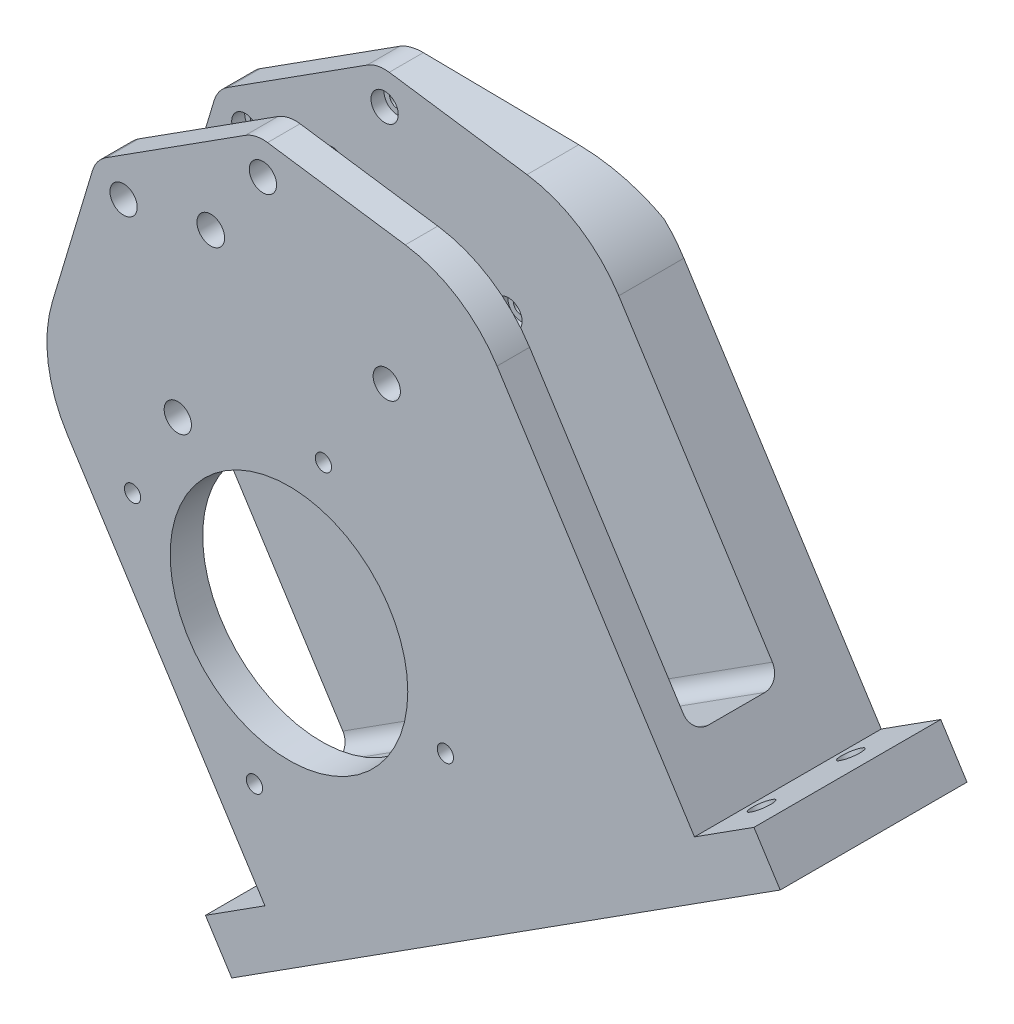
SolidWorks part; units mm, degrees
ref_plane "前视基准面" through (0, 0, 0) normal (0, 0, 1) x (1, 0, 0)
ref_plane "上视基准面" through (0, 0, 0) normal (0, 1, 0) x (1, 0, 0)
ref_plane "右视基准面" through (0, 0, 0) normal (1, 0, 0) x (0, 0, -1)
sketch "草图1" plane through (0, 0, 0) normal (0, 0, 1) x (1, 0, 0)
  line L0 (-42.8083, -27.3512) -> (0, 0) construction
  line L1 (-60.0492, -98.6503) -> (71.9432, -14.3176) construction
  line L2 (-21.4042, -13.6756) -> (-0.9851, -45.6342) construction
  line L3 (-48.1924, -18.9243) -> (-5.3841, 8.4268)
  line L4 (1.4167, 9.8991) -> (43.7508, 3.8405)
  line L5 (-52.3863, -24.4768) -> (-64.6788, -65.4375)
  line L6 (-60.0492, -98.6503) -> (-22.3606, -157.6382)
  line L7 (-22.3606, -157.6382) -> (109.6318, -73.3054)
  line L8 (71.9432, -14.3176) -> (109.6318, -73.3054)
  arc A0 (-48.1924, -18.9243) -> (-52.3863, -24.4768) centre (-42.8083, -27.3512) ccw
  arc A1 (1.4167, 9.8991) -> (-5.3841, 8.4268) centre (0, 0) ccw
  circle A2 centre (-26.1593, -76.9973) radius 4.191 construction
  circle A3 centre (38.0532, -35.9706) radius 4.191 construction
  arc A4 (-64.6788, -65.4375) -> (-60.0492, -98.6503) centre (-26.1593, -76.9973) ccw
  arc A5 (71.9432, -14.3176) -> (43.7508, 3.8405) centre (38.0532, -35.9706) ccw
  circle A6 centre (0, 0) radius 4.191 construction
  circle A7 centre (-42.8083, -27.3512) radius 4.191 construction
  circle A8 centre (-26.1593, -76.9973) radius 4.191
  circle A9 centre (38.0532, -35.9706) radius 4.191
  circle A10 centre (0, 0) radius 4.191
  circle A11 centre (-42.8083, -27.3512) radius 4.191
  dimension "D2" = 70
  dimension "D1" = 10
extrude "凸台-拉伸1" add sketch "草图1" along normal blind 10
sketch "草图2" plane through (0, 0, 0) normal (0, 0, -1) x (-1, 0, 0)
  line L0 (26.1593, -76.9973) -> (-0.8581, -119.2832) construction
  line L1 (-0.8581, -119.2832) -> (-8.004, -114.7175) construction
  line L2 (60.0492, -98.6503) -> (22.3606, -157.6382) construction
  line L3 (-38.0532, -35.9706) -> (26.1593, -76.9973) construction
  line L4 (-5.9747, -56.5274) -> (-32.002, -97.2637) construction
  circle A0 centre (-8.004, -114.7175) radius 2.5
  dimension "D1" = 50.18
  dimension "D3" = 5
  dimension "D2" = 29.62
extrude "切除-拉伸1" cut sketch "草图2" against normal blind 10
sketch "草图3" plane through (65.0398, -101.7962, 0) normal (0.5384, -0.8427, 0) x (0.8427, 0.5384, 0)
  line L4 (-103.7167, 0) -> (52.9167, 0)
  line L5 (52.9167, 0) -> (52.9167, 10)
  line L6 (52.9167, 10) -> (-103.7167, 10)
  line L7 (-103.7167, 10) -> (-103.7167, 0)
  line L8 (-103.7167, 0) -> (52.9167, 0)
  line L9 (52.9167, 0) -> (52.9167, 10)
  line L10 (52.9167, 10) -> (-103.7167, 10)
  line L11 (-103.7167, 10) -> (-103.7167, 0)
  dimension "D1" = 0
extrude "凸台-拉伸2" add sketch "草图3" along normal up to surface (22.68 mm away)
sketch "草图4" plane through (0, 0, 10) normal (0, 0, 1) x (1, 0, 0)
  circle A0 centre (8.004, -114.7175) radius 36.51 construction
  circle A1 centre (8.004, -114.7175) radius 36.51
extrude "切除-拉伸2" cut sketch "草图4" against normal through all
hole_wizard "M6 螺纹孔1" positions "草图5" profile "草图6" tap size "M6" standard "GB" end condition through all
sketch "草图5" plane through (0, 0, 10) normal (0, 0, 1) x (1, 0, 0)
  point P0 (-2.5848, -162.7795)
  point P3 (-40.058, -104.1287)
  point P6 (56.066, -125.3063)
  point P9 (18.5928, -66.6555)
sketch "草图6" plane through (-2.5848, -162.7795, 10) normal (1, 0, 0) x (0, -1, 0)
  line L0 (0, 0) -> (0, 10)
  line L1 (0, 10) -> (2.5, 10)
  line L2 (2.5, 10) -> (2.5, 0)
  line L5 (2.5, 0) -> (0, 0)
  line L11 (0, -6.35) -> (0, 107.95) construction
  dimension "通孔螺纹孔钻头直径" = 5
  dimension "通孔螺纹孔钻头深度" = 10
cosmetic thread "孔螺蚊线1" parameters "D2"=6
cosmetic thread "孔螺蚊线2" parameters "D2"=6
cosmetic thread "孔螺蚊线3" parameters "D2"=6
cosmetic thread "孔螺蚊线4" parameters "D2"=6
sketch "草图7" plane through (-87.4004, -55.8419, 0) normal (-0.8427, -0.5384, 0) x (0, 0, 1)
  line L0 (0, -143.48) -> (10, -143.48) construction
  line L1 (10, 10) -> (0, 10) construction
  line L2 (-27.4, -41.275) -> (-27.4, -60.325) construction
  line L3 (-27.4, -143.48) -> (10, -143.48)
  line L4 (-27.4, 10) -> (-37.4, 10)
  line L5 (-27.4, 10) -> (-27.4, -143.48)
  line L6 (-37.4, 21.9318) -> (-37.4, 10)
  line L7 (-47.4, -41.275) -> (-47.4, -163.48)
  line L8 (-16.7625, 22.8337) -> (-64.5437, 20.7455)
  line L9 (-37.4, -41.275) -> (-37.4, -60.325) construction
  line L10 (-27.4, -41.275) -> (-27.4, -60.325) construction
  line L11 (-37.4, 10) -> (-47.4, -41.275)
  line L13 (-47.4, -41.275) -> (-47.4, -60.325) construction
  line L14 (-47.4, -163.48) -> (10, -163.48)
  line L15 (10, -143.48) -> (10, -163.48)
  line L16 (-47.4, -143.48) -> (10, -143.48) construction
  dimension "D1" = 10
  dimension "D2" = 10
  dimension "D3" = 20
extrude "凸台-拉伸3" add sketch "草图7" against normal up to surface (156.6333 mm away) contours L11 L7 L14 L15 L3 L5 L4 up to face at (96.893, -53.3675, 5)
sketch "草图8" plane through (0, 0, -27.4) normal (0, 0, 1) x (1, 0, 0)
  line L0 (121.8429, -92.4175) -> (39.2079, 36.9176) construction
  line L1 (-92.7845, -47.4151) -> (-10.1495, -176.7502) construction
  line L2 (-52.3863, -24.4768) -> (-64.6788, -65.4375) construction
  line L3 (-5.3841, 8.4268) -> (-48.1924, -18.9243) construction
  line L4 (43.7508, 3.8405) -> (1.4167, 9.8991) construction
  line L5 (71.9432, -14.3176) -> (39.2079, 36.9176)
  line L6 (-92.7845, -47.4151) -> (-60.0492, -98.6503)
  line L7 (-52.3863, -24.4768) -> (-64.6788, -65.4375)
  line L8 (-5.3841, 8.4268) -> (-48.1924, -18.9243)
  line L9 (43.7508, 3.8405) -> (1.4167, 9.8991)
  line L10 (39.2079, 36.9176) -> (-7.9897, 44.9811)
  line L11 (-7.9897, 44.9811) -> (-89.9614, -17.3974)
  line L12 (-89.9614, -17.3974) -> (-92.7845, -47.4151)
  arc A0 (-64.6788, -65.4375) -> (-60.0492, -98.6503) centre (-26.1593, -76.9973) ccw construction
  arc A1 (-48.1924, -18.9243) -> (-52.3863, -24.4768) centre (-42.8083, -27.3512) ccw construction
  arc A2 (1.4167, 9.8991) -> (-5.3841, 8.4268) centre (0, 0) ccw construction
  arc A3 (71.9432, -14.3176) -> (43.7508, 3.8405) centre (38.0532, -35.9706) ccw construction
  arc A4 (-64.6788, -65.4375) -> (-60.0492, -98.6503) centre (-26.1593, -76.9973) ccw
  arc A5 (-48.1924, -18.9243) -> (-52.3863, -24.4768) centre (-42.8083, -27.3512) ccw
  arc A6 (1.4167, 9.8991) -> (-5.3841, 8.4268) centre (0, 0) ccw
  arc A7 (71.9432, -14.3176) -> (43.7508, 3.8405) centre (38.0532, -35.9706) ccw
extrude "切除-拉伸3" cut sketch "草图8" against normal through all
sketch "草图10" plane through (0, 0, -27.4) normal (0, 0, 1) x (1, 0, 0)
  circle A0 centre (38.0532, -35.9706) radius 4.191 construction
  circle A1 centre (-26.1593, -76.9973) radius 4.191 construction
  circle A2 centre (-42.8083, -27.3512) radius 4.191 construction
  circle A3 centre (0, 0) radius 4.191 construction
  circle A4 centre (38.0532, -35.9706) radius 4.191
  circle A5 centre (-26.1593, -76.9973) radius 4.191
  circle A6 centre (-42.8083, -27.3512) radius 4.191
  circle A7 centre (0, 0) radius 4.191
extrude "切除-拉伸4" cut sketch "草图10" against normal blind 4
hole_wizard "M6 螺纹孔2" positions "草图11" profile "草图12" tap size "M6" standard "GB" end condition through all
sketch "草图11" plane through (0, 0, -31.4) normal (0, 0, 1) x (1, 0, 0)
  point P0 (0, 0)
  point P3 (38.0532, -35.9706)
  point P6 (-26.1593, -76.9973)
  point P9 (-42.8083, -27.3512)
sketch "草图12" plane through (0, 0, -31.4) normal (1, 0, 0) x (0, -1, 0)
  line L0 (0, 0) -> (0, 16)
  line L1 (0, 16) -> (2.5, 16)
  line L2 (2.5, 16) -> (2.5, 0)
  line L5 (2.5, 0) -> (0, 0)
  line L11 (0, -6.35) -> (0, 107.95) construction
  dimension "通孔螺纹孔钻头直径" = 5
  dimension "通孔螺纹孔钻头深度" = 16
cosmetic thread "孔螺蚊线5" parameters "D2"=6
cosmetic thread "孔螺蚊线6" parameters "D2"=6
cosmetic thread "孔螺蚊线7" parameters "D2"=6
cosmetic thread "孔螺蚊线8" parameters "D2"=6
fillet "圆角2" radius 5 2 edges at (55.8467, -134.5839, 0) (55.8467, -134.5839, -27.4)
sketch "草图13" plane through (0, 0, 10) normal (0, 0, 1) x (1, 0, 0)
  line L0 (132.6111, -109.2712) -> (0.6187, -193.6039) construction
  line L1 (150.8833, -97.5967) -> (-17.6535, -205.2784)
  line L2 (158.9594, -110.2369) -> (-9.5774, -217.9187)
  line L3 (66.6149, -151.4375) -> (74.691, -164.0778)
  line L4 (-17.6535, -205.2784) -> (-9.5774, -217.9187)
  line L5 (150.8833, -97.5967) -> (158.9594, -110.2369)
  line L6 (132.6111, -109.2712) -> (0.6187, -193.6039) construction
  line L7 (140.6872, -121.9114) -> (8.6948, -206.2442) construction
  dimension "D2" = 100
  dimension "D1" = 15
  dimension "D3" = 100
extrude "凸台-拉伸4" add sketch "草图13" against normal up to surface (57.4 mm away) contours L2 L4 L1 L5 up to face at (40.5532, -35.9706, -47.4)
sketch "草图14" plane through (0, 0, 0) normal (0, 0, -1) x (-1, 0, 0)
  circle A0 centre (16.0201, -22.1024) radius 4.25 construction
  circle A1 centre (16.0201, -22.1024) radius 4.25
extrude "切除-拉伸5" cut sketch "草图14" against normal through all
hole_wizard "M8 螺纹孔1" positions "草图15" profile "草图16" tap size "M8" standard "GB" end condition through all
sketch "草图15" plane through (0, 0, -27.4) normal (0, 0, 1) x (1, 0, 0)
  point P0 (-16.0201, -22.1024)
sketch "草图16" plane through (-16.0201, -22.1024, -27.4) normal (1, 0, 0) x (0, -1, 0)
  line L0 (0, 0) -> (0, 20)
  line L1 (0, 20) -> (3.4, 20)
  line L2 (3.4, 20) -> (3.4, 0)
  line L5 (3.4, 0) -> (0, 0)
  line L11 (0, -6.35) -> (0, 107.95) construction
  dimension "通孔螺纹孔钻头直径" = 6.8
  dimension "通孔螺纹孔钻头深度" = 20
cosmetic thread "孔螺蚊线9" parameters "D2"=8
hole_wizard "M8 螺纹孔2" positions "草图17" profile "草图18" tap size "M8" standard "GB"
sketch "草图17" plane through (96.0952, -150.4022, 0) normal (0.5384, -0.8427, 0) x (-0.8427, -0.5384, 0)
  point P0 (110.4, 5)
  point P3 (110.4, 32.4)
  point P6 (-59.6, 32.4)
  point P9 (-59.6, 5)
sketch "草图18" plane through (3.0629, -209.8425, -5) normal (0, 0, 1) x (0.8427, 0.5384, 0)
  line L0 (0, 0) -> (0, 21.7929)
  line L1 (0, 21.7929) -> (3.4, 19.75)
  line L2 (3.4, 19.75) -> (3.4, 0)
  line L5 (3.4, 0) -> (0, 0)
  line L10 (0, 21.7929) -> (-3.4, 19.75) construction
  line L11 (0, -6.35) -> (0, 107.95) construction
  dimension "螺纹孔钻头直径" = 6.8
  dimension "螺纹孔钻头深度" = 19.75
  dimension "导头角度" = 118
cosmetic thread "孔螺蚊线10" parameters "D1"=15, "D2"=8
cosmetic thread "孔螺蚊线11" parameters "D1"=15, "D2"=8
cosmetic thread "孔螺蚊线12" parameters "D1"=15, "D2"=8
cosmetic thread "孔螺蚊线13" parameters "D1"=15, "D2"=8
hole_wizard "大小mm 暗销孔1" positions "草图19" profile "草图20" hole size "Ø10.0" standard "GB"
sketch "草图19" plane through (96.0952, -150.4022, 0) normal (0.5384, -0.8427, 0) x (-0.8427, -0.5384, 0)
  point P0 (65.4, 18.7)
  point P3 (-14.6, 18.7)
sketch "草图20" plane through (40.9836, -185.6141, -18.7) normal (0, 0, 1) x (0.8427, 0.5384, 0)
  line L0 (0, 0) -> (0, 22.7543)
  line L1 (0, 22.7543) -> (5, 19.75)
  line L2 (5, 19.75) -> (5, 0)
  line L5 (5, 0) -> (0, 0)
  line L10 (0, 22.7543) -> (-5, 19.75) construction
  line L11 (0, -6.35) -> (0, 107.95) construction
  dimension "孔直径" = 10
  dimension "孔深度" = 19.75
  dimension "导头角度" = 118
